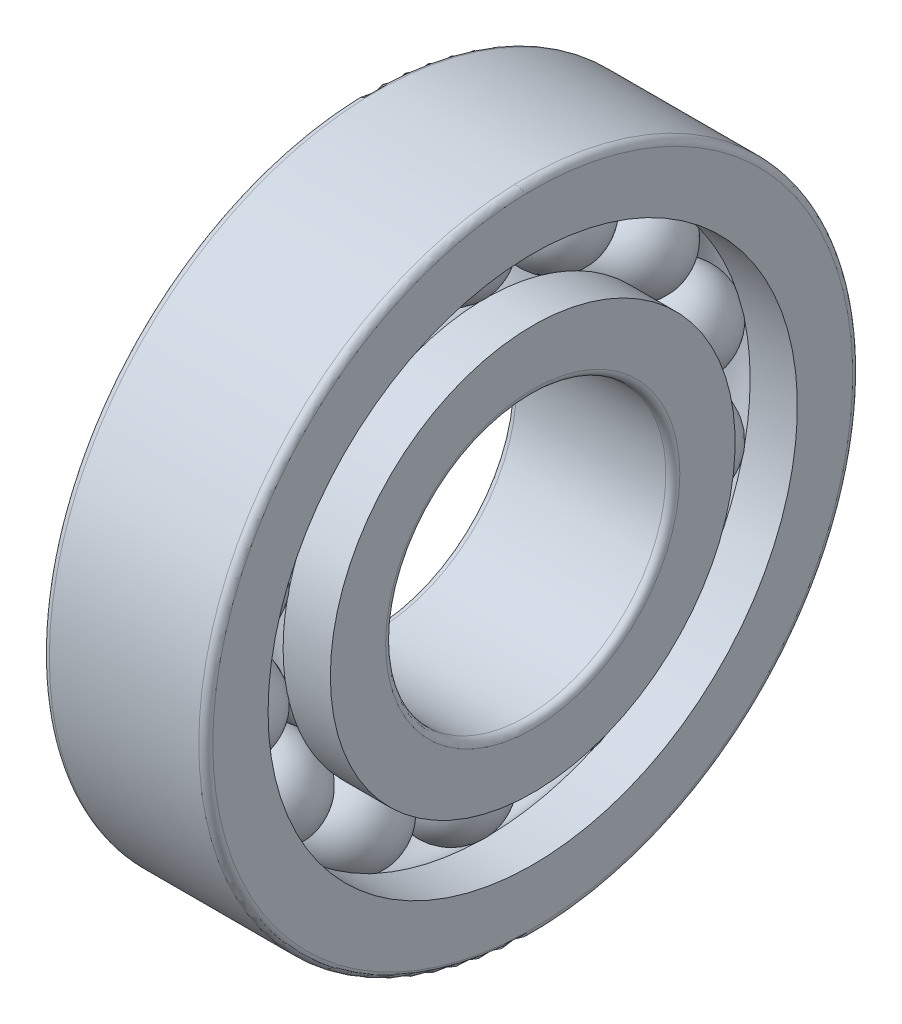
SolidWorks part; units mm, degrees
ref_plane "Front" through (0, 0, 0) normal (0, 0, 1) x (1, 0, 0)
ref_plane "Top" through (0, 0, 0) normal (0, 1, 0) x (1, 0, 0)
ref_plane "Right" through (0, 0, 0) normal (1, 0, 0) x (0, 0, -1)
sketch "Sketch1" plane through (0, 0, 0) normal (0, 0, 1) x (1, 0, 0)
  line L0 (-9.6833, 0) -> (9.8371, 0) construction
  line L1 (-2, 10) -> (2, 10)
  line L2 (-4.5966, 10) -> (4.6657, 10) construction
  arc A0 (2, 10) -> (-2, 10) centre (0, 10) ccw
revolve "Revolve1" add sketch "Sketch1" angle 360 about L2
sketch "Sketch2" plane through (0, 0, 0) normal (0, 0, 1) x (1, 0, 0)
  line L0 (-3.5, 8.6667) -> (-3.5, 6)
  line L1 (-3.5, 6) -> (3.5, 6)
  line L2 (3.5, 6) -> (3.5, 8.6667)
  line L3 (3.5, 8.6667) -> (1.4773, 8.6667)
  line L4 (-6.9714, 0) -> (8.1665, 0) construction
  line L5 (-6.7058, 10) -> (6.7058, 10) construction
  line L6 (-1.4773, 8.6667) -> (-3.5, 8.6667)
  arc A0 (-1.4773, 8.6667) -> (1.4773, 8.6667) centre (0, 10) ccw
revolve "Revolve2" add sketch "Sketch2" angle 360 about L4
sketch "Sketch3" plane through (0, 0, 0) normal (0, 0, 1) x (1, 0, 0)
  line L0 (-8.7107, 0) -> (9.1288, 0) construction
  line L1 (-3.5, 14) -> (3.5, 14)
  line L2 (-3.5, 14) -> (-3.5, 11.3333)
  line L3 (-3.5, 11.3333) -> (-1.4773, 11.3333)
  line L4 (3.5, 14) -> (3.5, 11.3333)
  line L5 (-7.2948, 10) -> (7.2948, 10) construction
  line L6 (1.4773, 11.3333) -> (3.5, 11.3333)
  arc A0 (1.4773, 11.3333) -> (-1.4773, 11.3333) centre (0, 10) ccw
revolve "Revolve3" add sketch "Sketch3" angle 360 about L0
pattern_circular "Circular-Pattern1" count 14 over 360 about axis through (0, 0, 0) along (1, 0, 0) of "Revolve1"
fillet "Fillet1" radius 0.3 4 edges at (-3.5, 0, 6) (-3.5, 0, 14) (3.5, 0, 14) (3.5, 0, 6)
equation "\"d0@Sketch1\" = ( \"DD@Sketch3\" + \"d@Sketch2\" )  / 2"
equation "\"dia@Sketch1\" =  ( \"DD@Sketch3\" - \"d@Sketch2\" )  / 4"
equation "\"D3@Sketch2\" = ( \"DD@Sketch3\" + \"d@Sketch2\" )  / 2 / 2"
equation "\"D4@Sketch2\" = ( \"DD@Sketch3\" - \"d@Sketch2\" )  / 6"
equation "\"D5@Sketch2\" = \"dia@Sketch1\" - 0.02"
equation "\"B/2@Sketch2\" = \"B@Sketch2\" / 2"
equation "\"D4@Sketch3\" = ( \"DD@Sketch3\" + \"d@Sketch2\" )  / 2 / 2"
equation "\"D5@Sketch3\" = ( \"DD@Sketch3\" - \"d@Sketch2\" )  / 6"
equation "\"B@Sketch3\" = \"B@Sketch2\""
equation "\"B/2@Sketch3\" = \"B@Sketch3\" / 2"
equation "\"D1@Sketch3\" = \"dia@Sketch1\" - 0.02"
equation "\"m@Circular-Pattern1\" = int( 3.14159265 / atn(( \"dia@Sketch1\" / 2) / sqr(( \"DD@Sketch3\" + \"d@Sketch2\" )  / 2 * ( \"DD@Sketch3\" + \"d@Sketch2\" )  / 2/4 - ( \"dia@Sketch1\" / 2) *  ( \"dia@Sketch1\" / 2))))-1"
